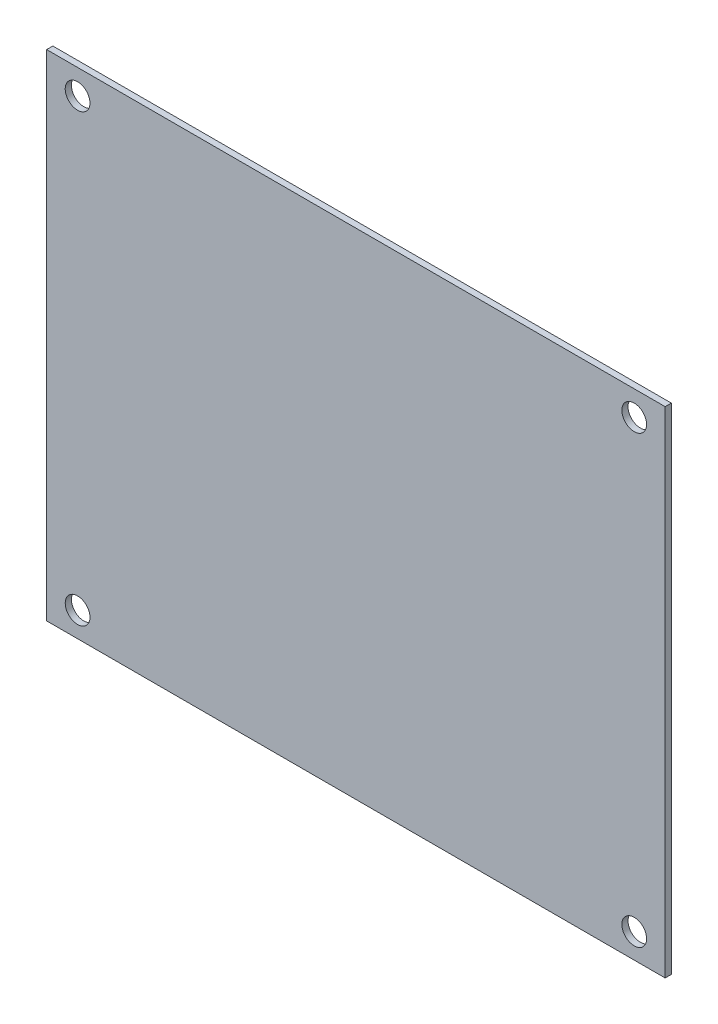
SolidWorks part; units mm, degrees
ref_plane "Front Plane" through (0, 0, 0) normal (0, 0, 1) x (1, 0, 0)
ref_plane "Top Plane" through (0, 0, 0) normal (0, 1, 0) x (1, 0, 0)
ref_plane "Right Plane" through (0, 0, 0) normal (1, 0, 0) x (0, 0, -1)
sketch "Sketch1" plane through (0, 0, 0) normal (0, 0, 1) x (1, 0, 0)
  line L0 (-45, 36) -> (45, 36) construction
  line L1 (-50, 40) -> (50, 40)
  line L2 (-50, 40) -> (-50, -40)
  line L3 (-50, -40) -> (50, -40)
  line L4 (50, 40) -> (50, -40)
  line L5 (-50, 40) -> (50, -40) construction
  line L6 (-50, -40) -> (50, 40) construction
  line L7 (0, 0) -> (35.7744, 0) construction
  line L8 (-45, -36) -> (45, -36) construction
  circle A1 centre (45, 36) radius 2
  circle A2 centre (-45, 36) radius 2
  circle A3 centre (-45, -36) radius 2
  circle A4 centre (45, -36) radius 2
  point P0 (0, 0)
  dimension "D3" = 5
  dimension "D1" = 80
  dimension "D2" = 100
  dimension "D4" = 5
  dimension "D5" = 4
extrude "Boss-Extrude1" add sketch "Sketch1" along normal blind 1
